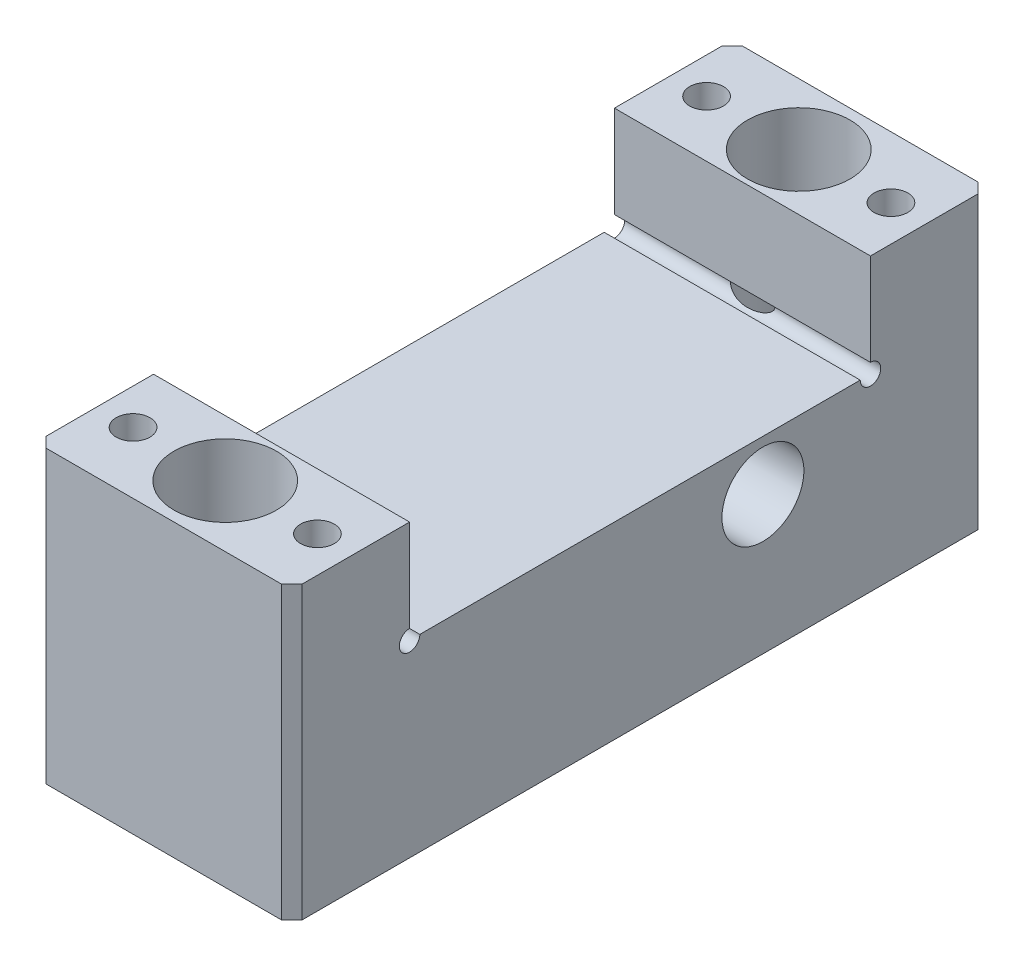
SolidWorks part; units mm, degrees
material "S45C"
ref_plane "前视基准面" through (0, 0, 0) normal (0, 0, 1) x (1, 0, 0)
ref_plane "上视基准面" through (0, 0, 0) normal (0, 1, 0) x (1, 0, 0)
ref_plane "右视基准面" through (0, 0, 0) normal (1, 0, 0) x (0, 0, -1)
sketch "草图1" plane through (0, 0, 0) normal (0, 1, 0) x (1, 0, 0)
  line L1 (-12.5, 34) -> (12.5, 34)
  line L2 (-12.5, 34) -> (-12.5, -34)
  line L3 (-12.5, -34) -> (12.5, -34)
  line L4 (12.5, 34) -> (12.5, -34)
  line L5 (-12.5, 34) -> (12.5, -34) construction
  line L6 (-12.5, -34) -> (12.5, 34) construction
  point P0 (0, 0)
  dimension "D1" = 68
  dimension "D2" = 25
extrude "凸台-拉伸1" add sketch "草图1" along normal mid plane 28.4
sketch "草图2" plane through (0, 14.2, 0) normal (0, 1, 0) x (1, 0, 0)
  line L0 (12.5, -34) -> (12.5, 34) construction
  line L1 (-12.5, 22.5) -> (12.5, 22.5)
  line L2 (-12.5, 22.5) -> (-12.5, -22.5)
  line L3 (-12.5, -22.5) -> (12.5, -22.5)
  line L4 (12.5, 22.5) -> (12.5, -22.5)
  line L5 (-12.5, 22.5) -> (12.5, -22.5) construction
  line L6 (-12.5, -22.5) -> (12.5, 22.5) construction
  point P0 (0, 0)
  dimension "D1" = 45
extrude "切除-拉伸1" cut sketch "草图2" against normal blind 10 and the other way through all
sketch "草图3" plane through (0, -14.2, 0) normal (0, -1, 0) x (-1, 0, 0)
  line L0 (0, 0) -> (25.0971, 0) construction
  point P0 (0, 15)
  point P7 (0, -15)
  dimension "D1" = 15
hole_wizard "Ø6.0mm 暗销孔1" positions "草图3" profile "草图4" hole size "Ø6.0" standard "ISO"
sketch "草图4" plane through (0, -14.2, -15) normal (1, 0, 0) x (0, 0, -1)
  line L0 (0, 0) -> (0, 7)
  line L1 (0, 7) -> (3, 7)
  line L2 (3, 7) -> (3, 0)
  line L5 (3, 0) -> (0, 0)
  line L10 (0, 7) -> (-3, 7) construction
  line L11 (0, -6.35) -> (0, 107.95) construction
  dimension "孔直径" = 6
  dimension "孔深度" = 7
  dimension "导头角度" = 180
sketch "草图5" plane through (0, 14.2, 0) normal (0, 1, 0) x (1, 0, 0)
  line L0 (0, 0) -> (30.5088, 0) construction
  line L1 (12.5, 34) -> (-12.5, 34) construction
  point P0 (0, 28)
  point P10 (0, -28)
  dimension "D1" = 6
hole_wizard "M5 六角凹头螺钉的柱形沉头孔1" positions "草图5" profile "草图6" counterbore size "M5" standard "ISO" end condition through all
sketch "草图6" plane through (0, 14.2, -28) normal (1, 0, 0) x (0, 0, 1)
  line L0 (0, 0) -> (0, 28.4)
  line L1 (0, 28.4) -> (2.75, 28.4)
  line L3 (2.75, 28.4) -> (2.75, 20)
  line L4 (2.75, 20) -> (5, 20)
  line L5 (5, 20) -> (5, 0)
  line L7 (5, 0) -> (0, 0)
  line L11 (0, -6.35) -> (0, 107.95) construction
  dimension "通孔孔直径" = 5.5
  dimension "通孔孔深度" = 28.4
  dimension "柱形沉头孔直径" = 10
  dimension "柱形沉头孔深度" = 20
sketch "草图7" plane through (0, 14.2, 0) normal (0, 1, 0) x (1, 0, 0)
  line L0 (0, 0) -> (0, -37.4258) construction
  line L1 (0, 0) -> (-30.4716, 0) construction
  line L2 (-12.5, -34) -> (12.5, -34) construction
  line L3 (-12.5, -22.5) -> (-12.5, -34) construction
  point P0 (-9, -28)
  point P14 (9, -28)
  point P15 (9, 28)
  point P16 (-9, 28)
  dimension "D1" = 6
  dimension "D2" = 3.5
hole_wizard "M4 螺纹孔1" positions "草图7" profile "草图8" tap size "M4" standard "ISO"
sketch "草图8" plane through (-9, 14.2, 28) normal (1, 0, 0) x (0, 0, 1)
  line L0 (0, 0) -> (0, 11.0914)
  line L1 (0, 11.0914) -> (1.65, 10.1)
  line L2 (1.65, 10.1) -> (1.65, 0)
  line L5 (1.65, 0) -> (0, 0)
  line L10 (0, 11.0914) -> (-1.65, 10.1) construction
  line L11 (0, -6.35) -> (0, 107.95) construction
  dimension "螺纹孔钻头直径" = 3.3
  dimension "螺纹孔钻头深度" = 10.1
  dimension "导头角度" = 118
cosmetic thread "孔螺蚊线1" parameters "D1"=8, "D2"=4
cosmetic thread "孔螺蚊线2" parameters "D1"=8, "D2"=4
cosmetic thread "孔螺蚊线3" parameters "D1"=8, "D2"=4
cosmetic thread "孔螺蚊线4" parameters "D1"=8, "D2"=4
chamfer "倒角1" distance 1 angle 45 4 edges at (-12.5, 0, -34) (12.5, 0, -34) (-12.5, 0, 34) (12.5, 0, 34)
sketch "草图9" plane through (-12.5, 0, 0) normal (-1, 0, 0) x (0, 0, 1)
  line L0 (-33, -14.2) -> (33, -14.2) construction
  circle A0 centre (-12, -0.7) radius 4
  dimension "D3" = 8
  dimension "D1" = 13.5
  dimension "D2" = 12
extrude "切除-拉伸2" cut sketch "草图9" against normal through all
sketch "草图10" plane through (12.5, 0, 0) normal (1, 0, 0) x (0, 0, -1)
  circle A0 centre (-22.5, 4.2) radius 1
  circle A1 centre (22.5, 4.2) radius 1
  dimension "D1" = 2
extrude "切除-拉伸3" cut sketch "草图10" against normal through all
